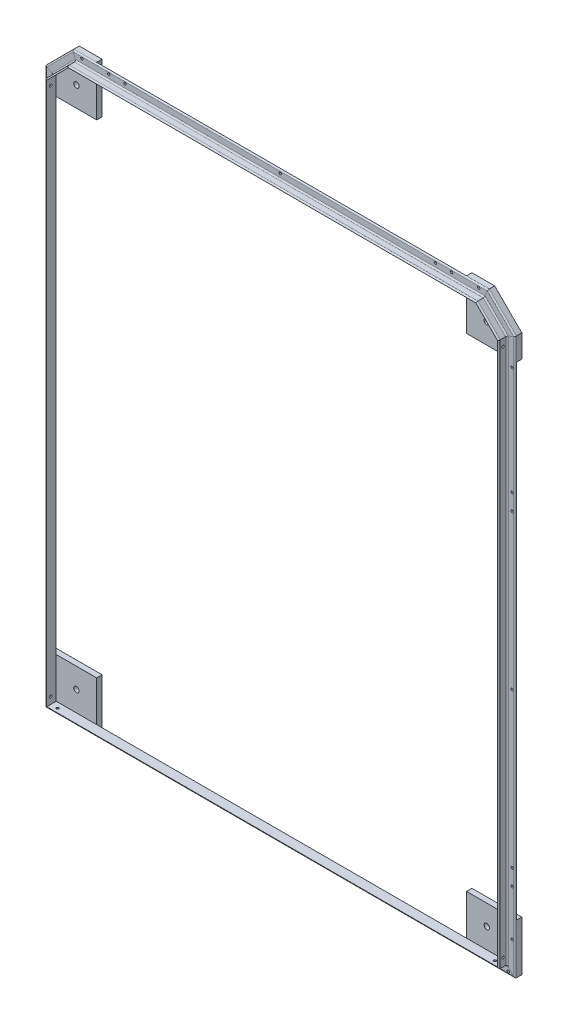
from build123d import *

# Parameters (mm, degrees)
MEMBER_1_DEPTH           = 2031.502525317
MEMBER_1_DEPTH_BACK      = 50.497474683
MEMBER_1_2_DEPTH         = 156.142135624
MEMBER_1_3_DEPTH         = 1553.005050634
MEMBER_1_4_DEPTH         = 156.142135624
MEMBER_1_5_DEPTH         = 2082
MEMBER_1_6_DEPTH         = 1770.994949366
SKETCH_3_R               = 10
EXTRUDE_1_DEPTH          = 20
SKETCH_3_W               = 185
SKETCH_3_H               = 185
EXTRUDE_1_2_DEPTH        = 20
EXTRUDE_1_3_DEPTH        = 20
EXTRUDE_1_4_DEPTH        = 20
SKETCH_4_R               = 4.5
CUT_EXTRUDE_1_DEPTH      = 10
CUT_EXTRUDE_2_DEPTH      = 2262
CUT_EXTRUDE_2_DEPTH_BACK = 328
SKETCH_5_R               = 4.5
SKETCH_6_R               = 4.5
CUT_EXTRUDE_3_DEPTH      = 236
SKETCH_7_R               = 4.5
CUT_EXTRUDE_4_DEPTH      = 228
SKETCH_8_R               = 4.5
CUT_EXTRUDE_5_DEPTH      = 99
SKETCH_9_R               = 4.5
CUT_EXTRUDE_6_DEPTH      = 78


with BuildPart() as part:
    # Sketch1 → Member 1 (new, two sides: drawn at the far end of the back side and taken through both)
    with BuildSketch(Plane(origin=(0, 0, 0), x_dir=(-1, 0, 0), z_dir=(0, 1, 0)).offset(-MEMBER_1_DEPTH_BACK)):
        with BuildLine():
            Line((0, 0), (0, 35))
            ThreePointArc((0, 35), (3.535533906, 33.535533906), (5, 30))
            Line((5, 30), (5, 10))
            ThreePointArc((5, 10), (6.464466094, 6.464466094), (10, 5))
            Line((10, 5), (30, 5))
            ThreePointArc((30, 5), (33.535533906, 3.535533906), (35, 0))
            Line((35, 0), (0, 0))
        make_face()
    extrude(amount=MEMBER_1_DEPTH + MEMBER_1_DEPTH_BACK)

    # Member 1 mitre 1
    split(bisect_by=Plane(origin=(0, 0, 0), x_dir=(-0.707106781, -0.707106781, 0), z_dir=(-0.707106781, 0.707106781, 0)), keep=Keep.TOP)

    # Member 1 mitre 2
    split(bisect_by=Plane(origin=(0, 2010, 0), x_dir=(0.923879533, -0.382683432, 0), z_dir=(-0.382683432, -0.923879533, 0)), keep=Keep.TOP)


with BuildPart() as body_2:
    # Sketch1 on segment 2 (carried to segment 2) → Member 1 2 (new body)
    with BuildSketch(Plane(origin=(-15.204581464, 1994.795418536, 0), x_dir=(-0.707106781, 0.707106781, 0), z_dir=(0.707106781, 0.707106781, 0))):
        with BuildLine():
            Line((0, 0), (0, 35))
            ThreePointArc((0, 35), (3.535533906, 33.535533906), (5, 30))
            Line((5, 30), (5, 10))
            ThreePointArc((5, 10), (6.464466094, 6.464466094), (10, 5))
            Line((10, 5), (30, 5))
            ThreePointArc((30, 5), (33.535533906, 3.535533906), (35, 0))
            Line((35, 0), (0, 0))
        make_face()
    extrude(amount=MEMBER_1_2_DEPTH)

    # Member 1 2 mitre 1
    split(bisect_by=Plane(origin=(0, 2010, 0), x_dir=(-0.923879533, 0.382683432, 0), z_dir=(0.382683432, 0.923879533, 0)), keep=Keep.TOP)

    # Member 1 2 mitre 2
    split(bisect_by=Plane(origin=(80, 2090, 0), x_dir=(0.382683432, -0.923879533, 0), z_dir=(-0.923879533, -0.382683432, 0)), keep=Keep.TOP)


with BuildPart() as body_3:
    # Sketch1 on segment 3 (carried to segment 3) → Member 1 3 (new body)
    with BuildSketch(Plane(origin=(58.497474683, 2090, 0), x_dir=(0, 1, 0), z_dir=(1, 0, 0))):
        with BuildLine():
            Line((0, 0), (0, 35))
            ThreePointArc((0, 35), (3.535533906, 33.535533906), (5, 30))
            Line((5, 30), (5, 10))
            ThreePointArc((5, 10), (6.464466094, 6.464466094), (10, 5))
            Line((10, 5), (30, 5))
            ThreePointArc((30, 5), (33.535533906, 3.535533906), (35, 0))
            Line((35, 0), (0, 0))
        make_face()
    extrude(amount=MEMBER_1_3_DEPTH)

    # Member 1 3 mitre 1
    split(bisect_by=Plane(origin=(80, 2090, 0), x_dir=(-0.382683432, 0.923879533, 0), z_dir=(0.923879533, 0.382683432, 0)), keep=Keep.TOP)

    # Member 1 3 mitre 2
    split(bisect_by=Plane(origin=(1590, 2090, 0), x_dir=(-0.382683432, -0.923879533, 0), z_dir=(-0.923879533, 0.382683432, 0)), keep=Keep.TOP)


with BuildPart() as body_4:
    # Sketch1 on segment 4 (carried to segment 4) → Member 1 4 (new body)
    with BuildSketch(Plane(origin=(1574.795418536, 2105.204581464, 0), x_dir=(0.707106781, 0.707106781, 0), z_dir=(0.707106781, -0.707106781, 0))):
        with BuildLine():
            Line((0, 0), (0, 35))
            ThreePointArc((0, 35), (3.535533906, 33.535533906), (5, 30))
            Line((5, 30), (5, 10))
            ThreePointArc((5, 10), (6.464466094, 6.464466094), (10, 5))
            Line((10, 5), (30, 5))
            ThreePointArc((30, 5), (33.535533906, 3.535533906), (35, 0))
            Line((35, 0), (0, 0))
        make_face()
    extrude(amount=MEMBER_1_4_DEPTH)

    # Member 1 4 mitre 1
    split(bisect_by=Plane(origin=(1590, 2090, 0), x_dir=(0.382683432, 0.923879533, 0), z_dir=(0.923879533, -0.382683432, 0)), keep=Keep.TOP)

    # Member 1 4 mitre 2
    split(bisect_by=Plane(origin=(1670, 2010, 0), x_dir=(-0.923879533, -0.382683432, 0), z_dir=(-0.382683432, 0.923879533, 0)), keep=Keep.TOP)


with BuildPart() as body_5:
    # Sketch1 on segment 5 (carried to segment 5) → Member 1 5 (new body)
    with BuildSketch(Plane(origin=(1670, 2031.502525317, 0), x_dir=(1, 0, 0), z_dir=(0, -1, 0))):
        with BuildLine():
            Line((0, 0), (0, 35))
            ThreePointArc((0, 35), (3.535533906, 33.535533906), (5, 30))
            Line((5, 30), (5, 10))
            ThreePointArc((5, 10), (6.464466094, 6.464466094), (10, 5))
            Line((10, 5), (30, 5))
            ThreePointArc((30, 5), (33.535533906, 3.535533906), (35, 0))
            Line((35, 0), (0, 0))
        make_face()
    extrude(amount=MEMBER_1_5_DEPTH)

    # Member 1 5 mitre 1
    split(bisect_by=Plane(origin=(1670, 0, 0), x_dir=(-0.707106781, 0.707106781, 0), z_dir=(0.707106781, 0.707106781, 0)), keep=Keep.TOP)

    # Member 1 5 mitre 2
    split(bisect_by=Plane(origin=(1670, 2010, 0), x_dir=(0.923879533, 0.382683432, 0), z_dir=(0.382683432, -0.923879533, 0)), keep=Keep.TOP)


with BuildPart() as body_6:
    # Sketch1 on segment 6 (carried to segment 6) → Member 1 6 (new body)
    with BuildSketch(Plane(origin=(1720.497474683, 0, 0), x_dir=(0, -1, 0), z_dir=(-1, 0, 0))):
        with BuildLine():
            Line((0, 0), (0, 35))
            ThreePointArc((0, 35), (3.535533906, 33.535533906), (5, 30))
            Line((5, 30), (5, 10))
            ThreePointArc((5, 10), (6.464466094, 6.464466094), (10, 5))
            Line((10, 5), (30, 5))
            ThreePointArc((30, 5), (33.535533906, 3.535533906), (35, 0))
            Line((35, 0), (0, 0))
        make_face()
    extrude(amount=MEMBER_1_6_DEPTH)

    # Member 1 6 mitre 1
    split(bisect_by=Plane(origin=(0, 0, 0), x_dir=(0.707106781, 0.707106781, 0), z_dir=(0.707106781, -0.707106781, 0)), keep=Keep.TOP)

    # Member 1 6 mitre 2
    split(bisect_by=Plane(origin=(1670, 0, 0), x_dir=(0.707106781, -0.707106781, 0), z_dir=(-0.707106781, -0.707106781, 0)), keep=Keep.TOP)

    # 草图4 → 切除-拉伸1 (cut)
    with BuildSketch(Plane(origin=(0, 0, 0), x_dir=(1, 0, 0), z_dir=(0, 1, 0))):
        with Locations(Location((25, -20, 0), (0, 0, 270))):
            Circle(SKETCH_4_R)
        with Locations(Location((1645, -20, 0), (0, 0, 270))):
            Circle(SKETCH_4_R)
    extrude(amount=-CUT_EXTRUDE_1_DEPTH, mode=Mode.SUBTRACT)


with BuildPart() as body_7:
    # 草图3 → 凸台-拉伸1 (new body)
    with BuildSketch(Plane(origin=(0, 0, 0), x_dir=(-1, 0, 0), z_dir=(0, 0, -1))):
        Polygon((-1604.497474683, 2125), (-1705, 2024.497474683), (-1705, 1940), (-1520, 1940), (-1520, 2125), align=None)
        with Locations((-1595, 2015)):
            Circle(SKETCH_3_R, mode=Mode.SUBTRACT)
    extrude(amount=EXTRUDE_1_DEPTH)


with BuildPart() as body_8:
    # 草图3 → Extrude 1 2 (new body)
    with BuildSketch(Plane(origin=(0, 0, 0), x_dir=(-1, 0, 0), z_dir=(0, 0, -1))):
        with Locations((-1612.5, 57.5)):
            Rectangle(SKETCH_3_W, SKETCH_3_H)
        with Locations((-1595, 75)):
            Circle(SKETCH_3_R, mode=Mode.SUBTRACT)
    extrude(amount=EXTRUDE_1_2_DEPTH)


with BuildPart() as body_9:
    # 草图3 → Extrude 1 3 (new body)
    with BuildSketch(Plane(origin=(0, 0, 0), x_dir=(-1, 0, 0), z_dir=(0, 0, -1))):
        with Locations((-57.5, 57.5)):
            Rectangle(SKETCH_3_W, SKETCH_3_H)
        with Locations(Location((-75, 75, 0), (0, 0, 180))):
            Circle(SKETCH_3_R, mode=Mode.SUBTRACT)
    extrude(amount=EXTRUDE_1_3_DEPTH)


with BuildPart() as body_10:
    # 草图3 → Extrude 1 4 (new body)
    with BuildSketch(Plane(origin=(0, 0, 0), x_dir=(-1, 0, 0), z_dir=(0, 0, -1))):
        Polygon((-150, 2125), (-65.502525317, 2125), (35, 2024.497474683), (35, 1940), (-150, 1940), align=None)
        with Locations(Location((-75, 2015, 0), (0, 0, 180))):
            Circle(SKETCH_3_R, mode=Mode.SUBTRACT)
    extrude(amount=EXTRUDE_1_4_DEPTH)


with BuildPart() as cut_extrude_2_tool:
    # 草图5 → 切除-拉伸2 (new, two sides: drawn at the far end of the back side and taken through both)
    with BuildSketch(Plane(origin=(0, 0, 0), x_dir=(0, 0, -1), z_dir=(1, 0, 0)).offset(-CUT_EXTRUDE_2_DEPTH_BACK)):
        with Locations(Location((-20, 25, 0), (0, 0, 180))):
            Circle(SKETCH_5_R)
        with Locations(Location((-20, 1985, 0), (0, 0, 180))):
            Circle(SKETCH_5_R)
    extrude(amount=CUT_EXTRUDE_2_DEPTH + CUT_EXTRUDE_2_DEPTH_BACK)


with BuildPart() as part_1:
    add(part.part)

    # 切除-拉伸2: cut by cut_extrude_2_tool
    add(cut_extrude_2_tool.part, mode=Mode.SUBTRACT)


with BuildPart() as body_5_1:
    add(body_5.part)

    # 切除-拉伸2: cut by cut_extrude_2_tool
    add(cut_extrude_2_tool.part, mode=Mode.SUBTRACT)


with BuildPart() as cut_extrude_3_tool:
    # 草图6 → 切除-拉伸3 (new body)
    with BuildSketch(Plane.XY.offset(5)):
        with Locations((100, 2114)):
            Circle(SKETCH_6_R)
        with Locations((200, 2114)):
            Circle(SKETCH_6_R)
        with Locations((-24, 1920)):
            Circle(SKETCH_6_R)
        with Locations((-24, 1790)):
            Circle(SKETCH_6_R)
        with Locations((1470, 2114)):
            Circle(SKETCH_6_R)
        with Locations((1570, 2114)):
            Circle(SKETCH_6_R)
        with Locations((1694, 1920)):
            Circle(SKETCH_6_R)
        with Locations((1694, 1519)):
            Circle(SKETCH_6_R)
        with Locations((260, 2114)):
            Circle(SKETCH_6_R)
        with Locations((835, 2114)):
            Circle(SKETCH_6_R)
        with Locations((1410, 2114)):
            Circle(SKETCH_6_R)
    extrude(amount=-CUT_EXTRUDE_3_DEPTH)


with BuildPart() as part_2:
    add(part_1.part)

    # 切除-拉伸3: cut by cut_extrude_3_tool
    add(cut_extrude_3_tool.part, mode=Mode.SUBTRACT)


with BuildPart() as body_3_1:
    add(body_3.part)

    # 切除-拉伸3: cut by cut_extrude_3_tool
    add(cut_extrude_3_tool.part, mode=Mode.SUBTRACT)


with BuildPart() as body_5_2:
    add(body_5_1.part)

    # 切除-拉伸3: cut by cut_extrude_3_tool
    add(cut_extrude_3_tool.part, mode=Mode.SUBTRACT)


with BuildPart() as body_7_1:
    add(body_7.part)

    # 切除-拉伸3: cut by cut_extrude_3_tool
    add(cut_extrude_3_tool.part, mode=Mode.SUBTRACT)


with BuildPart() as body_10_1:
    add(body_10.part)

    # 切除-拉伸3: cut by cut_extrude_3_tool
    add(cut_extrude_3_tool.part, mode=Mode.SUBTRACT)


with BuildPart() as cut_extrude_4_tool:
    # 草图7 → 切除-拉伸4 (new body)
    with BuildSketch(Plane.XY.offset(5)):
        with Locations((-24, 73)):
            Circle(SKETCH_7_R)
        with Locations((-24, 273)):
            Circle(SKETCH_7_R)
        with Locations((80, -24)):
            Circle(SKETCH_7_R)
    extrude(amount=-CUT_EXTRUDE_4_DEPTH)


with BuildPart() as part_3:
    add(part_2.part)

    # 切除-拉伸4: cut by cut_extrude_4_tool
    add(cut_extrude_4_tool.part, mode=Mode.SUBTRACT)


with BuildPart() as body_6_1:
    add(body_6.part)

    # 切除-拉伸4: cut by cut_extrude_4_tool
    add(cut_extrude_4_tool.part, mode=Mode.SUBTRACT)


with BuildPart() as body_9_1:
    add(body_9.part)

    # 切除-拉伸4: cut by cut_extrude_4_tool
    add(cut_extrude_4_tool.part, mode=Mode.SUBTRACT)


with BuildPart() as cut_extrude_5_tool:
    # 草图8 → 切除-拉伸5 (new body)
    with BuildSketch(Plane.XY.offset(5)):
        with Locations((1694, 255)):
            Circle(SKETCH_8_R)
        with Locations((1694, 85)):
            Circle(SKETCH_8_R)
        with Locations((1694, 315)):
            Circle(SKETCH_8_R)
        with Locations((1694, 887)):
            Circle(SKETCH_8_R)
        with Locations((1694, 1459)):
            Circle(SKETCH_8_R)
    extrude(amount=-CUT_EXTRUDE_5_DEPTH)


with BuildPart() as body_5_3:
    add(body_5_2.part)

    # 切除-拉伸5: cut by cut_extrude_5_tool
    add(cut_extrude_5_tool.part, mode=Mode.SUBTRACT)


with BuildPart() as body_8_1:
    add(body_8.part)

    # 切除-拉伸5: cut by cut_extrude_5_tool
    add(cut_extrude_5_tool.part, mode=Mode.SUBTRACT)


with BuildPart() as cut_extrude_6_tool:
    # 草图9 → 切除-拉伸6 (new body)
    with BuildSketch(Plane.XY.offset(5)):
        with Locations((1680, -24)):
            Circle(SKETCH_9_R)
        with Locations((140, -24)):
            Circle(SKETCH_9_R)
        with Locations((910, -24)):
            Circle(SKETCH_9_R)
    extrude(amount=-CUT_EXTRUDE_6_DEPTH)


with BuildPart() as body_6_2:
    add(body_6_1.part)

    # 切除-拉伸6: cut by cut_extrude_6_tool
    add(cut_extrude_6_tool.part, mode=Mode.SUBTRACT)


with BuildPart() as body_8_2:
    add(body_8_1.part)

    # 切除-拉伸6: cut by cut_extrude_6_tool
    add(cut_extrude_6_tool.part, mode=Mode.SUBTRACT)


with BuildPart() as body_9_2:
    add(body_9_1.part)

    # 切除-拉伸6: cut by cut_extrude_6_tool
    add(cut_extrude_6_tool.part, mode=Mode.SUBTRACT)


solid = Compound([body_2.part, body_4.part, body_3_1.part, body_7_1.part, body_10_1.part, part_3.part, body_5_3.part, body_6_2.part, body_8_2.part, body_9_2.part])
